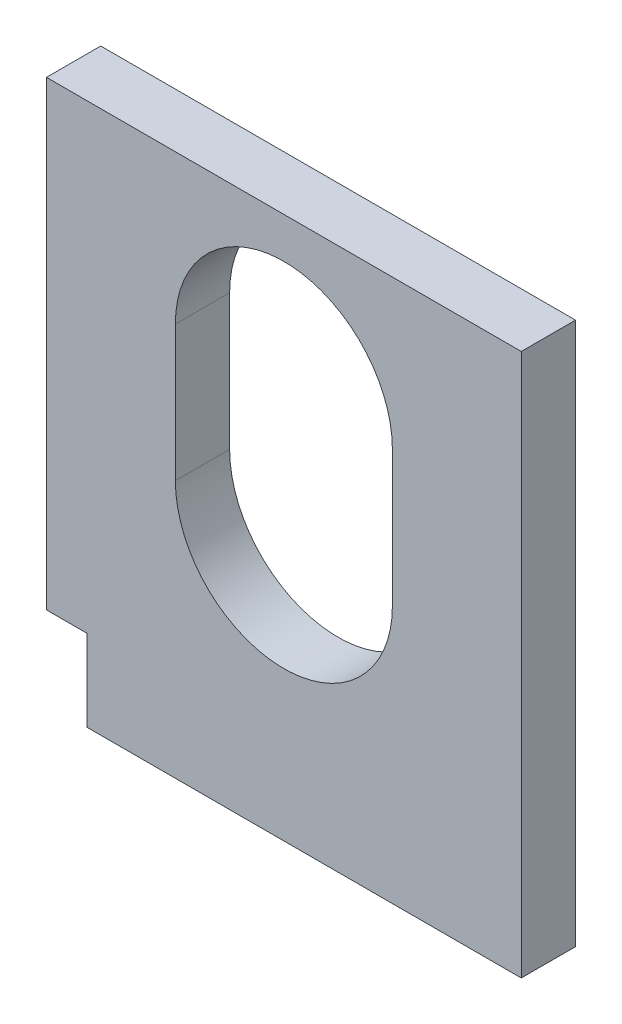
SolidWorks part; units mm, degrees
ref_plane "Front Plane" through (0, 0, 0) normal (0, 0, 1) x (1, 0, 0)
ref_plane "Top Plane" through (0, 0, 0) normal (0, 1, 0) x (1, 0, 0)
ref_plane "Right Plane" through (0, 0, 0) normal (1, 0, 0) x (0, 0, -1)
sketch "Sketch1" plane through (0, 0, 0) normal (0, 0, 1) x (1, 0, 0)
  line L1 (3, 0) -> (35, 0)
  line L2 (0, 5.9978) -> (0, 40)
  line L3 (0, 40) -> (35, 40)
  line L4 (35, 0) -> (35, 40)
  line L5 (9.5, 29) -> (9.5, 19)
  line L6 (25.5, 29) -> (25.5, 19)
  line L7 (19, 11.1419) -> (19, 0) construction
  line L8 (3, 5.9978) -> (3, 0)
  line L9 (0, 5.9978) -> (3, 5.9978)
  arc A0 (25.5, 29) -> (9.5, 29) centre (17.5, 29) ccw
  arc A1 (9.5, 19) -> (25.5, 19) centre (17.5, 19) ccw
  dimension "D4" = 10
  dimension "D5" = 16
  dimension "D6" = 16
  dimension "D7" = 5.9978
  dimension "D1" = 40
  dimension "D2" = 3
  dimension "D8" = 35
extrude "Boss-Extrude1" add sketch "Sketch1" along normal blind 4
